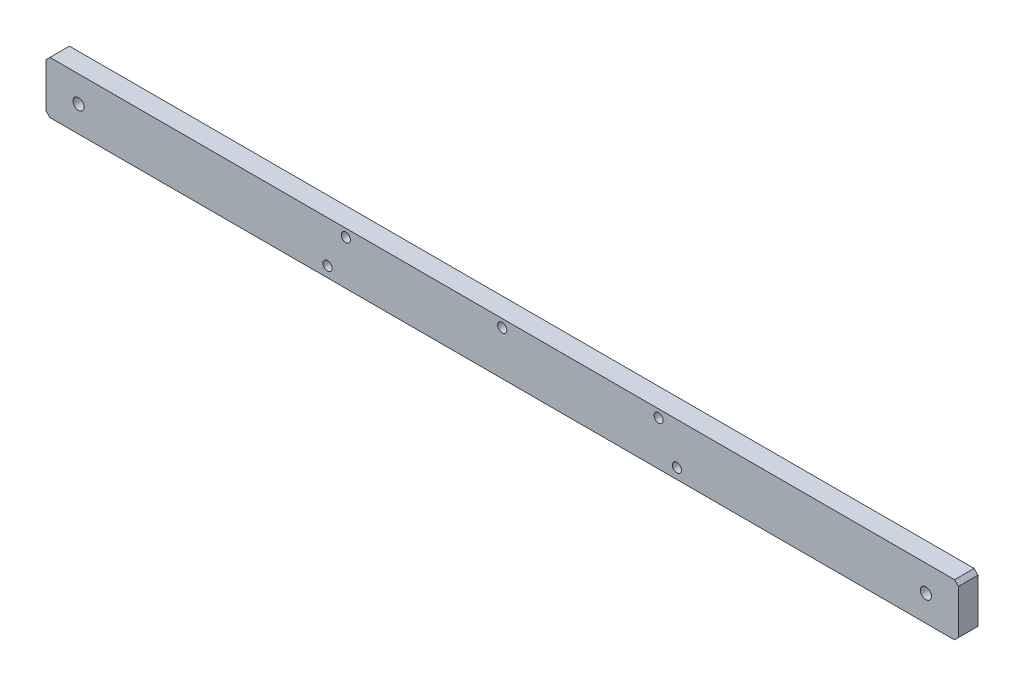
from build123d import *

# Parameters (mm, degrees)
SKETCH_1_W            = 700
SKETCH_1_H            = 40
EXTRUDE_1_DEPTH       = 15
CHAMFER_1_SIZE        = 3
HOLE_WIZARD_M10_1_D   = 8.5
HOLE_WIZARD_7_0_7_1_D = 7


with BuildPart() as part:
    # 草图1 → 凸台-拉伸1 (new body)
    with BuildSketch(Plane.XY):
        with Locations((350, -20)):
            Rectangle(SKETCH_1_W, SKETCH_1_H)
    extrude(amount=EXTRUDE_1_DEPTH)

    # 倒角1
    chamfer_1_edges = [part.edges().sort_by_distance(p)[0] for p in [
        (0, 0, 7.5),
        (700, 0, 7.5),
        (700, -40, 7.5),
        (0, -40, 7.5),
    ]]
    chamfer(chamfer_1_edges, length=CHAMFER_1_SIZE)

    # M10 螺纹孔1 (through all)
    with Locations(Plane.XY.offset(15)):
        with Locations((25, -20), (675, -20)):
            Hole(HOLE_WIZARD_M10_1_D / 2)

    # Ø7.0 (7) 直径孔1 (through all)
    with Locations(Plane.XY.offset(15)):
        with Locations((470, -6), (350, -6), (230, -6), (216, -32), (484, -32)):
            Hole(HOLE_WIZARD_7_0_7_1_D / 2)


solid = part.part
